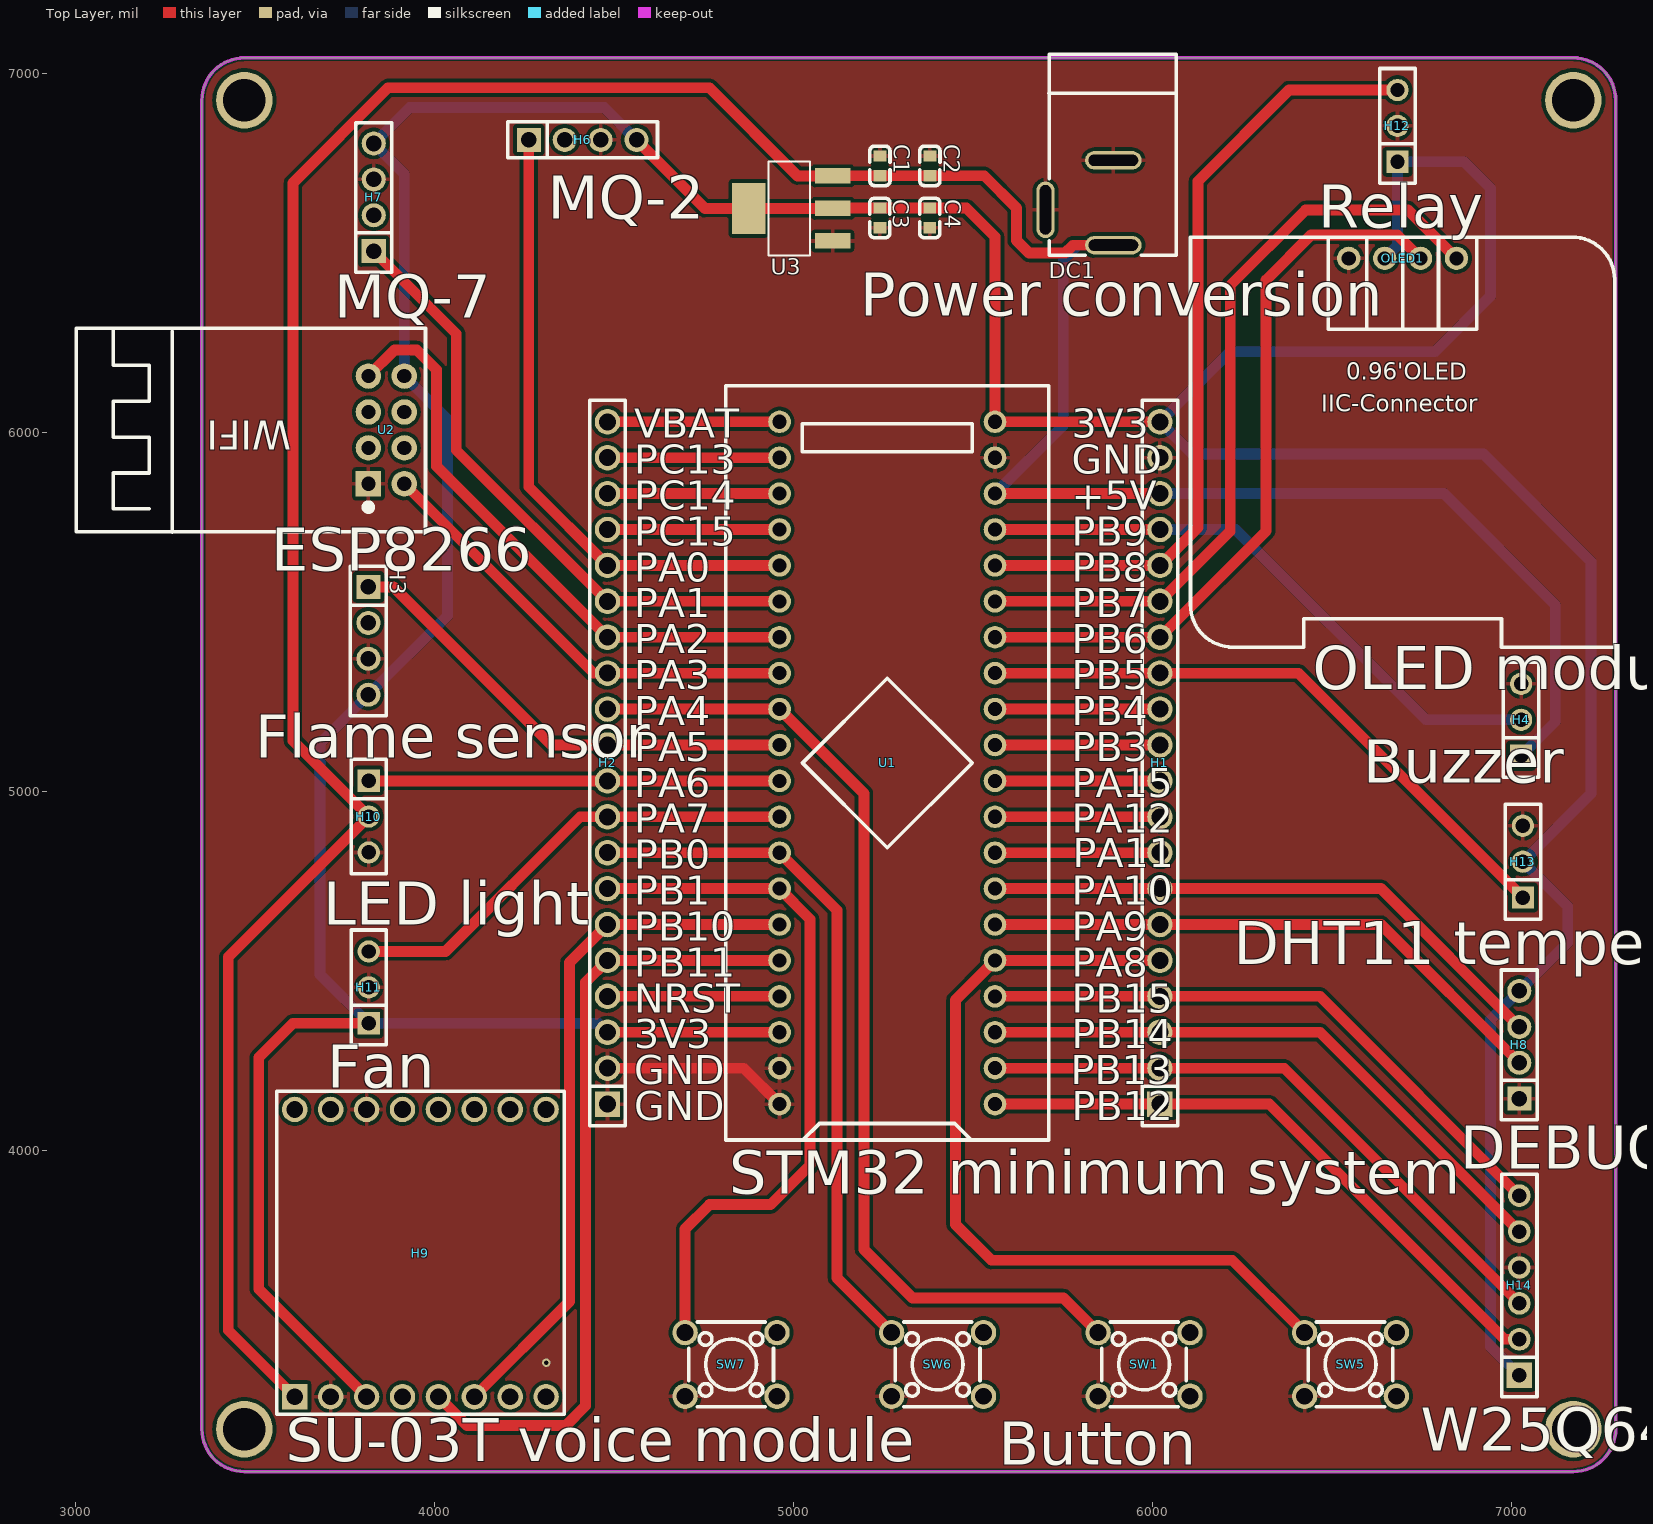
[diagram p0: Top Layer view]
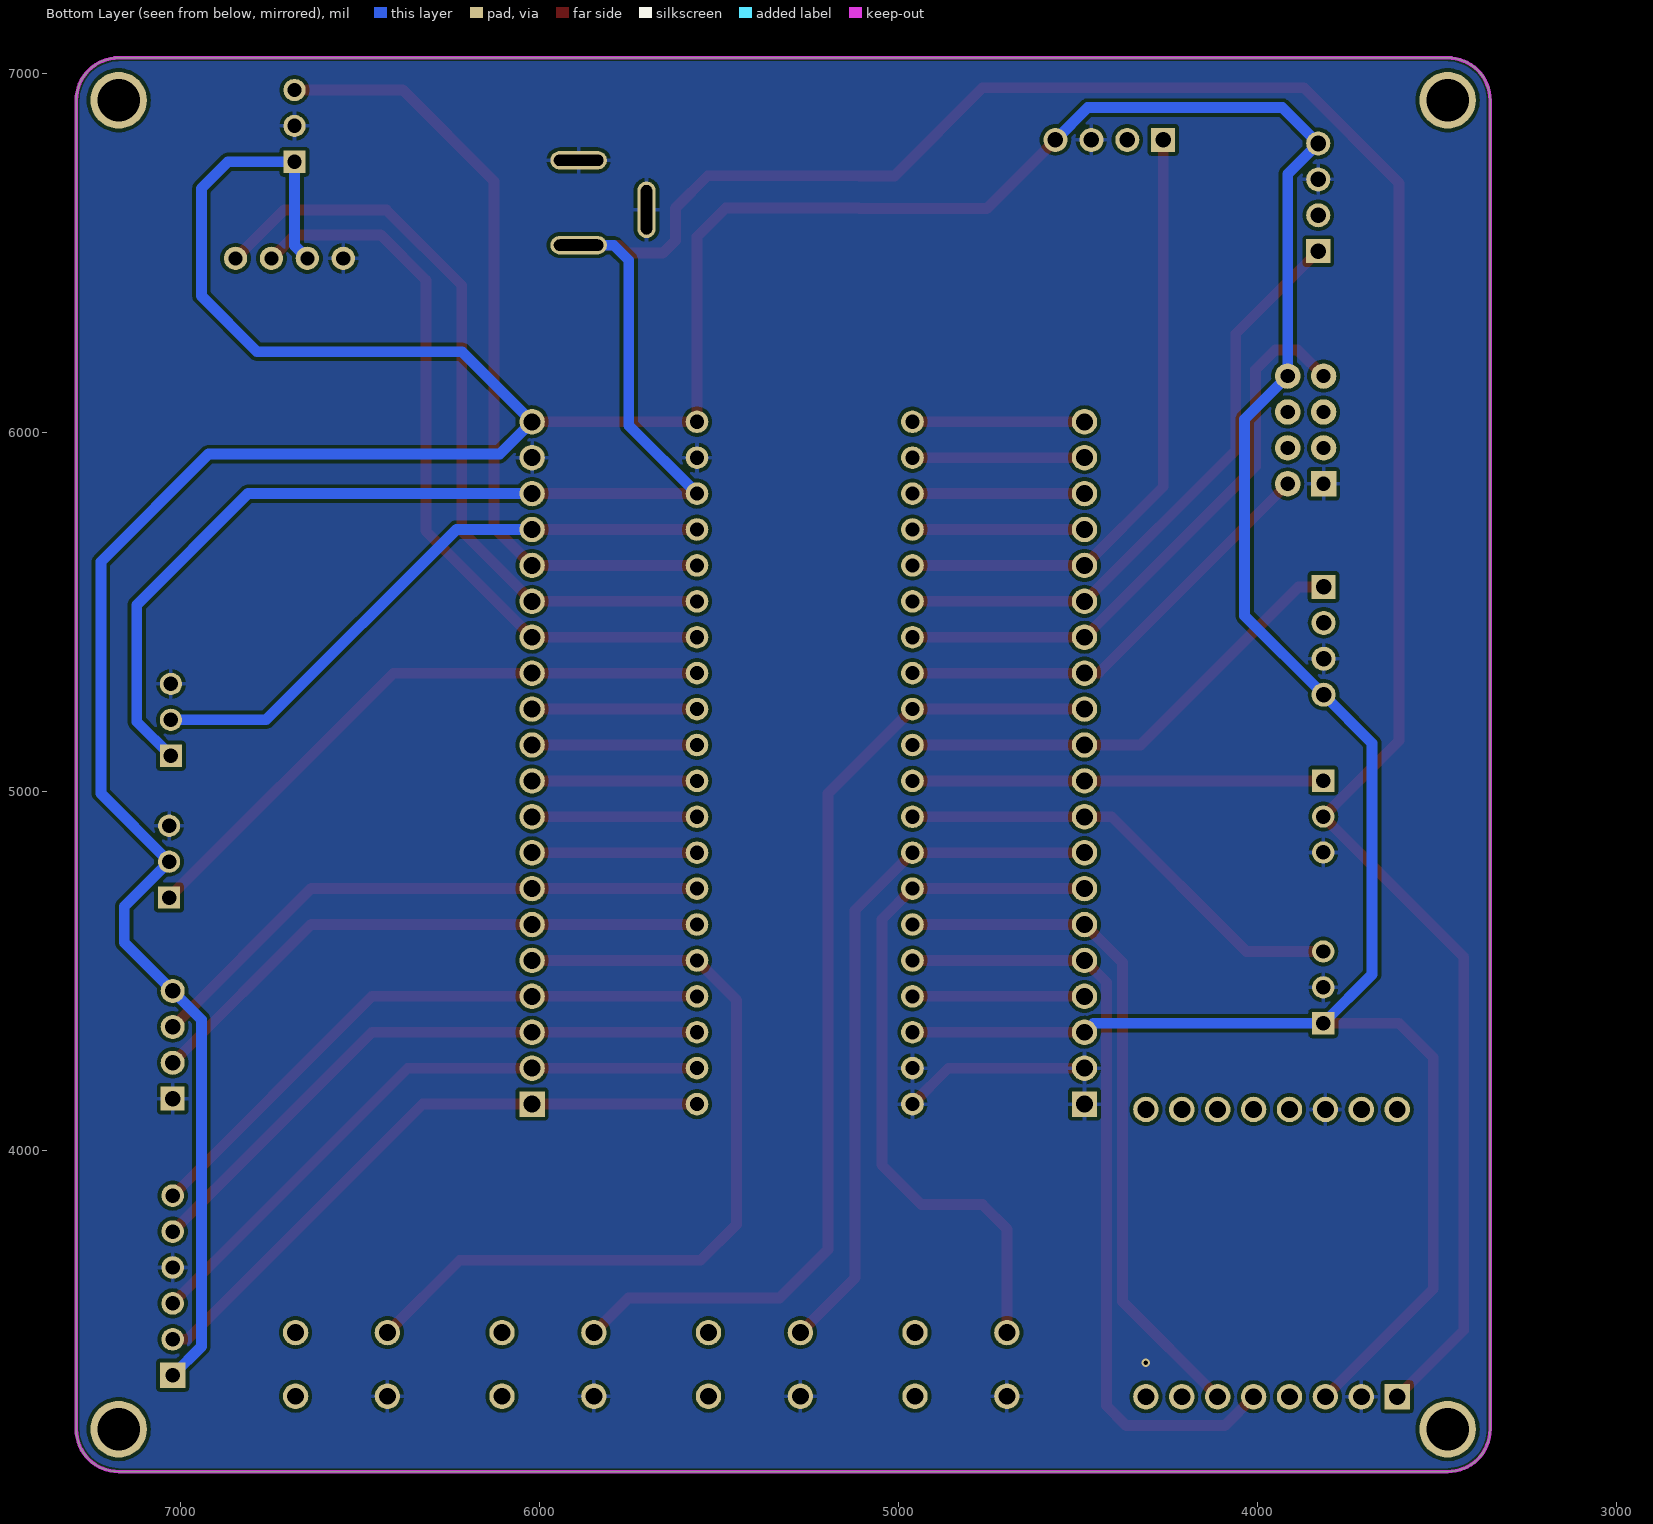
[diagram p1: Bottom Layer view, seen from below]
# Altium PCB MISC51915.pcbdoc
Units mil, origin at the board's own origin, x right, y up, seen from the top; angles counter-clockwise.
Board outline 3937.01 x 3937.01 mil, 2 copper layers (Top Layer, Bottom Layer), stack 62.206 mil thick; 26 components, 37 nets, 180 pads, 1 vias.

## Layer stack, top to bottom
Top Solder Mask Layer: solder mask 0.394, Dk 3.3
Top Layer: signal copper 1.379
Dielectric1: surface 59.449, FR4, Dk 4.5
Bottom Layer: signal copper 1.378
Bottom Solder Mask Layer: solder mask 0.394, Dk 3.3

## Board outline
3470.35,7043.5 ccw(c3470.35,6925.39) 3352.24,6925.39 3352.24,3224.61 ccw(c3470.35,3224.61) 3470.35,3106.5 7171.14,3106.5 ccw(c7171.14,3224.61) 7289.25,3224.61 7289.25,6925.39 ccw(c7171.14,6925.39) 7171.14,7043.5 3470.35,7043.5

## Design rules (kind name [scope] priority, off if disabled: settings)
BoardOutlineClearance copperThickness2oz_1 [All] p2 off: genericclearance=7.99 ignorepadtopadclearanceinfootprint=FALSE except(0: Arc-SplitContinuation Track-SplitContinuation SMDPad-SplitContinuation THPad-SplitContinuation Via-SplitContinuation Fill-SplitContinuation Region-SplitContinuation Poly-SplitContinuation Text-SplitContinuation Hole-SplitContinuation; 5.98: Arc-CutoutEdge Track-CutoutEdge SMDPad-CutoutEdge THPad-CutoutEdge Via-CutoutEdge Text-CutoutEdge; 6.9: Hole-OutlineEdge Hole-CutoutEdge; 10: Poly-OutlineEdge Poly-CutoutEdge; 11.81: Arc-OutlineEdge Track-OutlineEdge SMDPad-OutlineEdge THPad-OutlineEdge Via-OutlineEdge Fill-OutlineEdge Region-OutlineEdge Text-OutlineEdge Fill-CutoutEdge Region-CutoutEdge)
BoardOutlineClearance Plane_innerPlane_1 [All] p4 off: genericclearance=4.02 ignorepadtopadclearanceinfootprint=FALSE except(0: Arc-SplitContinuation Track-SplitContinuation SMDPad-SplitContinuation THPad-SplitContinuation Via-SplitContinuation Fill-SplitContinuation Region-SplitContinuation Poly-SplitContinuation Text-SplitContinuation Hole-SplitContinuation; 5.98: Arc-CutoutEdge Track-CutoutEdge SMDPad-CutoutEdge THPad-CutoutEdge Via-CutoutEdge Text-CutoutEdge; 6.9: Hole-OutlineEdge Hole-CutoutEdge; 10: Poly-OutlineEdge Poly-CutoutEdge; 11.81: Arc-OutlineEdge Track-OutlineEdge SMDPad-OutlineEdge THPad-OutlineEdge Via-OutlineEdge Fill-OutlineEdge Region-OutlineEdge Text-OutlineEdge Fill-CutoutEdge Region-CutoutEdge)
BoardOutlineClearance Copper_copperRegion_1 [All] p6 off: genericclearance=4.02 ignorepadtopadclearanceinfootprint=FALSE except(0: Arc-SplitContinuation Track-SplitContinuation SMDPad-SplitContinuation THPad-SplitContinuation Via-SplitContinuation Fill-SplitContinuation Region-SplitContinuation Poly-SplitContinuation Text-SplitContinuation Hole-SplitContinuation; 5.98: Arc-CutoutEdge Track-CutoutEdge SMDPad-CutoutEdge THPad-CutoutEdge Via-CutoutEdge Text-CutoutEdge; 6.9: Hole-OutlineEdge Hole-CutoutEdge; 10: Poly-OutlineEdge Poly-CutoutEdge; 11.81: Arc-OutlineEdge Track-OutlineEdge SMDPad-OutlineEdge THPad-OutlineEdge Via-OutlineEdge Fill-OutlineEdge Region-OutlineEdge Text-OutlineEdge Fill-CutoutEdge Region-CutoutEdge)
BoardOutlineClearance copperThickness1oz_1 [All] p8: genericclearance=4.02 ignorepadtopadclearanceinfootprint=FALSE except(0: Arc-SplitContinuation Track-SplitContinuation SMDPad-SplitContinuation THPad-SplitContinuation Via-SplitContinuation Fill-SplitContinuation Region-SplitContinuation Poly-SplitContinuation Text-SplitContinuation Hole-SplitContinuation; 5.98: Arc-CutoutEdge Track-CutoutEdge SMDPad-CutoutEdge THPad-CutoutEdge Via-CutoutEdge Text-CutoutEdge; 6.9: Hole-OutlineEdge Hole-CutoutEdge; 10: Poly-OutlineEdge Poly-CutoutEdge; 11.81: Arc-OutlineEdge Track-OutlineEdge SMDPad-OutlineEdge THPad-OutlineEdge Via-OutlineEdge Fill-OutlineEdge Region-OutlineEdge Text-OutlineEdge Fill-CutoutEdge Region-CutoutEdge)
Clearance copperThickness2oz [All] p1 off: gap=7.99 ignorepadtopadclearanceinfootprint=FALSE except(5.98: SMDPad-Track SMDPad-SMDPad THPad-Track SMDPad-THPad THPad-THPad Track-Via SMDPad-Via THPad-Via Via-Via Fill-SMDPad Region-SMDPad Fill-THPad Region-THPad Fill-Via Region-Via Fill-Fill Fill-Region Region-Region Arc-Track Arc-SMDPad Arc-THPad Arc-Via Fill-Arc Region-Arc Arc-Arc Text-Track SMDPad-Text Text-THPad Text-Via Fill-Text Region-Text Arc-Text Text-Text; 6.9: Hole-Track Hole-SMDPad Hole-THPad Hole-Via Fill-Hole Region-Hole Hole-Arc Hole-Text; 10: Poly-Track Poly-SMDPad Poly-THPad Poly-Via Poly-Fill Poly-Region Poly-Poly Poly-Arc Poly-Text Poly-Hole; 11.81: Fill-Track Region-Track)
Clearance Plane_innerPlane [All] p3 off: gap=4.02 ignorepadtopadclearanceinfootprint=FALSE except(5.98: SMDPad-Track SMDPad-SMDPad THPad-Track SMDPad-THPad THPad-THPad Track-Via SMDPad-Via THPad-Via Via-Via Fill-SMDPad Region-SMDPad Fill-THPad Region-THPad Fill-Via Region-Via Fill-Fill Fill-Region Region-Region Arc-Track Arc-SMDPad Arc-THPad Arc-Via Fill-Arc Region-Arc Arc-Arc Text-Track SMDPad-Text Text-THPad Text-Via Fill-Text Region-Text Arc-Text Text-Text; 6.9: Hole-Track Hole-SMDPad Hole-THPad Hole-Via Fill-Hole Region-Hole Hole-Arc Hole-Text; 10: Poly-Track Poly-SMDPad Poly-THPad Poly-Via Poly-Fill Poly-Region Poly-Poly Poly-Arc Poly-Text Poly-Hole; 11.81: Fill-Track Region-Track)
Clearance Copper_copperRegion [All] p5 off: gap=4.02 ignorepadtopadclearanceinfootprint=FALSE except(5.98: SMDPad-Track SMDPad-SMDPad THPad-Track SMDPad-THPad THPad-THPad Track-Via SMDPad-Via THPad-Via Via-Via Fill-SMDPad Region-SMDPad Fill-THPad Region-THPad Fill-Via Region-Via Fill-Fill Fill-Region Region-Region Arc-Track Arc-SMDPad Arc-THPad Arc-Via Fill-Arc Region-Arc Arc-Arc Text-Track SMDPad-Text Text-THPad Text-Via Fill-Text Region-Text Arc-Text Text-Text; 6.9: Hole-Track Hole-SMDPad Hole-THPad Hole-Via Fill-Hole Region-Hole Hole-Arc Hole-Text; 10: Poly-Track Poly-SMDPad Poly-THPad Poly-Via Poly-Fill Poly-Region Poly-Poly Poly-Arc Poly-Text Poly-Hole; 11.81: Fill-Track Region-Track)
Clearance copperThickness1oz [All] p7: gap=4.02 ignorepadtopadclearanceinfootprint=FALSE except(5.98: SMDPad-Track SMDPad-SMDPad THPad-Track SMDPad-THPad THPad-THPad Track-Via SMDPad-Via THPad-Via Via-Via Fill-SMDPad Region-SMDPad Fill-THPad Region-THPad Fill-Via Region-Via Fill-Fill Fill-Region Region-Region Arc-Track Arc-SMDPad Arc-THPad Arc-Via Fill-Arc Region-Arc Arc-Arc Text-Track SMDPad-Text Text-THPad Text-Via Fill-Text Region-Text Arc-Text Text-Text; 6.9: Hole-Track Hole-SMDPad Hole-THPad Hole-Via Fill-Hole Region-Hole Hole-Arc Hole-Text; 10: Poly-Track Poly-SMDPad Poly-THPad Poly-Via Poly-Fill Poly-Region Poly-Poly Poly-Arc Poly-Text Poly-Hole; 11.81: Fill-Track Region-Track)
DiffPairsRouting differentialPair [All] p1: maxlimit=6 minlimit=6 mostfreqgap=6 toplayer_minwidth=5 toplayer_prefwidth=10 toplayer_maxwidth=100 toplayer_mingap=6 toplayer_prefgap=6 toplayer_maxgap=6 bottomlayer_minwidth=5 bottomlayer_prefwidth=10 bottomlayer_maxwidth=100 bottomlayer_mingap=6 bottomlayer_prefgap=6 bottomlayer_maxgap=6 maxuncoupledlength=10
HoleToHoleClearance otherClearance [All] p1: gap=11.81 allowstackedmicrovias=TRUE
Length netLength [All] p1: minlimit=0 maxlimit=0
PasteMaskExpansion pasteMaskExpansion [All] p1: expansion=0
PlaneConnect innerPlane [All] p1: planeconnectstyle=Relief reliefexpansion=20 reliefentries=4 reliefconductorwidth=10 reliefairgap=10
PolygonConnect copperRegion [All] p1: connectstyle=Relief reliefconductorwidth=10 reliefentries=4 polygonreliefangle="90 Angle" airgapwidth=10 via.connectstyle=Relief via.reliefconductorwidth=10 via.reliefentries=4 via.polygonreliefangle="90 Angle" via.airgapwidth=10
RoutingVias viaSize [All] p1: holewidth=12.01 width=24.02 viastyle="Through Hole" minholewidth=11.81 minwidth=19.68 maxholewidth=248.03 maxwidth=393.7
SolderMaskExpansion solderMaskExpansion [IsVia] p1: expansion=-1000 istentingtop=TRUE
SolderMaskExpansion solderMaskExpansion [All] p2: expansion=2 istentingtop=FALSE
Width copperThickness2oz_2 [All] p1 off: maxlimit=100 minlimit=8 preferedwidth=10
Width copperThickness1oz_2 [All] p2: maxlimit=100 minlimit=5 preferedwidth=10

## Components (designator, comment, footprint, x,y, rotation, side; value= is the part's Value field where it differs from the comment)
C1 "100nF" C0603 5240.36,6742.51 r270 top
C2 "100nF" C0603 5379.49,6742.51 r270 top
C3 "100nF" C0603 5240.19,6597.5 r90 top
C4 "100nF" C0603 5379.32,6597.5 r90 top
DC1 "" DC-2.0 5900.75,6645 r90 top
H1 "" HDR-TH_20P-P2.54-V-F 6019.91,5080 r90 top
H2 "" HDR-TH_20P-P2.54-V-F 4481.7,5080 r90 top
H3 "" HDR-TH_4P-P2.54-V-F 3815.75,5420 r270 top
H4 "" HDR-TH_3P-P2.54-V-F 7025.75,5200 r90 top
H6 "" HDR-TH_4P-P2.54-V-F 4412.53,6815 r0 top
H7 "" HDR-TH_4P-P2.54-V-F 3830.75,6655 r90 top
H8 "" HDR-TH_4P-P2.54-V-F 7020.75,4295 r90 top
H9 "" HDR-TH_16P-P2.54-V-M-R2-C8-S2.54 3910.75,3315 r0 top
H10 "" HDR-TH_3P-P2.54-V-F 3816.75,4930.71 r270 top
H11 "" HDR-TH_3P-P2.54-V-F 3816.75,4455 r90 top
H12 "" HDR-TH_3P-P2.54-V-F 6681.51,6853.84 r90 top
H13 "" HDR-TH_3P-P2.54-V-F 7030.75,4805 r90 top
H14 "" HDR-TH_6P-P2.54-V-F 7020.75,3625 r90 top
OLED1 "" 0.96OLED_4P 6695.75,6485 r0 top
SW1 "" SW-TH_4P-L6.0-W6.0-P4.50-LS6.5 5975.75,3405 r0 top
SW5 "" SW-TH_4P-L6.0-W6.0-P4.50-LS6.5 6550.75,3405 r0 top
SW6 "" SW-TH_4P-L6.0-W6.0-P4.50-LS6.5 5400.75,3405 r0 top
SW7 "" SW-TH_4P-L6.0-W6.0-P4.50-LS6.5 4825.75,3405 r0 top
U1 "STM32F103C8T6-Card" CONN-TH_L53.3-W22.9_STM32F103C8T6-CARD 5260.75,5080 r90 top
U2 "Ai-Thinker ESP-01S ESP8266" WIFIM-TH_8P-L24.7-W14.4-P2.54 3865.75,6007.3 r180 top
U3 "AMS1117-3.3" SOT-223-3_L6.5-W3.4-P2.30-LS7.0-BR 4991.9,6624.1 r0 top

## Footprints (in the part's own frame and the unit in brackets; to place one, negate y for a bottom-side part, rotate by r counter-clockwise, add the part's x,y. Pads: shape width x height; smd on the part's side, far side on the other; paste and mask are expansions set on the pad)
0.96OLED_4P [mm]
  round 1.65 hole 1 copper offset 0,0: 1(-3.81,-0.001) 2(-1.27,0.002) 3(1.27,0.002) 4(3.81,0.002)
  silkscreen extent -15,-27.5 15,1.5
C0603 [mm]
  rect 0.8x0.9 smd: 1(-0.7,0) 2(0.7,0)
  silkscreen extent -1.39,-0.71 1.39,0.71
CONN-TH_L53.3-W22.9_STM32F103C8T6-CARD [mm]
  round 1.6 hole 1: 1(-24.13,-7.62) 2(-21.59,-7.62) 3(-19.05,-7.62) 4(-16.51,-7.62) 5(-13.97,-7.62) 6(-11.43,-7.62) 7(-8.89,-7.62) 8(-6.35,-7.62) 9(-3.81,-7.62) 10(-1.27,-7.62) 11(1.27,-7.62) 12(3.81,-7.62) 13(6.35,-7.62) 14(8.89,-7.62) 15(11.43,-7.62) 16(13.97,-7.62) 17(16.51,-7.62) 18(19.05,-7.62) 19(21.59,-7.62) 20(24.13,-7.62) 21(24.13,7.62) 22(21.59,7.62) 23(19.05,7.62) 24(16.51,7.62) 25(13.97,7.62) 26(11.43,7.62) 27(8.89,7.62) 28(6.35,7.62) 29(3.81,7.62) 30(1.27,7.62) 31(-1.27,7.62) 32(-3.81,7.62) 33(-6.35,7.62) 34(-8.89,7.62) 35(-11.43,7.62) 36(-13.97,7.62) 37(-16.51,7.62) 38(-19.05,7.62) 39(-21.59,7.62) 40(-24.13,7.62)
  silkscreen extent -26.67,-11.43 26.67,11.43
DC-2.0 [mil]
  oval 157.5x51.2 hole 31.5 slot 137.8 at 0 deg paste+0 mask+2: 2(-24.7,199.5)
  oval 51.2x157.5 hole 31.5 slot 137.8 at 90 deg paste+0 mask+2: 3(113.1,10.5) 4(-123.1,10.5)
  silkscreen extent -151,-165 408,190
HDR-TH_3P-P2.54-V-F [mil]
  rect 62x62 hole 40.16: 1(-100,0)
  round 62 hole 40.16: 2(0,0) 3(100,0)
  silkscreen extent -160,-49 160,49
HDR-TH_4P-P2.54-V-F [mm]
  rect 1.7x1.7 hole 1.1: 1(-3.81,0)
  round 1.7 hole 1.1: 2(-1.27,0) 3(1.27,0) 4(3.81,0)
  silkscreen extent -5.29,-1.27 5.29,1.27
HDR-TH_6P-P2.54-V-F [mm]
  rect 1.8x1.8 hole 1.02: 1(-6.35,0)
  round 1.6 hole 1.02: 2(-3.81,0) 3(-1.27,0) 4(1.27,0) 5(3.81,0) 6(6.35,0)
  silkscreen extent -7.87,-1.25 7.87,1.25
HDR-TH_16P-P2.54-V-M-R2-C8-S2.54 [mm]
  rect 1.8x1.8 hole 1.2: 1(-7.62,0)
  round 1.8 hole 1.2: 2(-7.62,20.32) 3(-5.08,0) 4(-5.08,20.32) 5(-2.54,0) 6(-2.54,20.32) 7(0,0) 8(0,20.32) 9(2.54,0) 10(2.54,20.32) 11(5.08,0) 12(5.08,20.32) 13(7.62,0) 14(7.62,20.32) 15(10.16,0) 16(10.16,20.32)
  silkscreen extent -8.89,-1.23 11.43,21.6
HDR-TH_20P-P2.54-V-F [mm]
  rect 1.8x1.8 hole 1.2: 1(-24.13,0)
  round 1.8 hole 1.2: 2(-21.59,0) 3(-19.05,0) 4(-16.51,0) 5(-13.97,0) 6(-11.43,0) 7(-8.89,0) 8(-6.35,0) 9(-3.81,0) 10(-1.27,0) 11(1.27,0) 12(3.81,0) 13(6.35,0) 14(8.89,0) 15(11.43,0) 16(13.97,0) 17(16.51,0) 18(19.05,0) 19(21.59,0) 20(24.13,0)
  silkscreen extent -25.65,-1.25 25.65,1.25
SOT-223-3_L6.5-W3.4-P2.30-LS7.0-BR [mm]
  rect 2.5x1.1 smd: 1(2.97,-2.3) 2(2.97,0) 3(2.97,2.3)
  rect 2.34x3.6 smd: 4(-2.97,0)
  silkscreen extent -1.57,-3.33 1.37,3.33
SW-TH_4P-L6.0-W6.0-P4.50-LS6.5 [mm]
  round 1.8 hole 1.2: 1(-3.25,2.25) 2(3.25,2.25) 3(-3.25,-2.25) 4(3.25,-2.25)
  silkscreen extent -3,-3 3,3
WIFIM-TH_8P-L24.7-W14.4-P2.54 [mm]
  rect 1.8x1.8 hole 1 paste+0 mask+0.05: 1(1.27,3.81)
  round 1.8 hole 1 paste+0 mask+0.05: 2(1.27,1.27) 3(1.27,-1.27) 4(1.27,-3.81) 5(-1.27,3.81) 6(-1.27,1.27) 7(-1.27,-1.27) 8(-1.27,-3.81)
  silkscreen extent -2.77,-7.19 21.93,7.24

## Free pads (board coordinates)
  round 157.48 hole 118.11: 1(3470.35,6925.39) 1(3470.35,3224.61) 1(7171.14,6925.39) 1(7171.14,3224.61)

## Via types
v1: diameter 24.02, hole 12, Top Layer to Bottom Layer, 1 vias

## Nets (pads, with @x,y where several pads share a name; then routed paths per layer and width w, separated by ;. In a path a pad name is that pad's centre, name@x,y a point inside that pad or via, vN(x,y) a via of type N, cw(c..) or ccw(c..) an arc to the next point about the centre after c; other vN are vias at no path point)
+5V: C1.2 C2.2 DC1.4 H1.18 H4.1 H9.1 H10.2 U1.18 U3.3 | length 9386.1
  Top Layer w30: H9.1 3425.75,3500 3425.75,4539.71 H10.2 3605.75,5141.71 3605.75,6695 3870.75,6960 4765.75,6960 5011.1,6714.65 U3.3 5109.12,6714.95 C1.2 C2.2 5530.8,6714.95 5620.75,6625 5620.75,6535 5655.75,6500 5755.75,6500 5777.65,6521.9 DC1.4 ; U1.18 H1.18
  Bottom Layer w30: U1.18 5750.75,6020 5750.75,6480 5792.65,6521.9 DC1.4 ; H1.18 6810.75,5830 7120.75,5520 7120.75,5195 H4.1
GND: C1.1 C2.1 C3.1 C4.1 DC1.2 DC1.3 H1.19 H2.1 H2.2 H3.3 H4.3 H6.3 H7.3 H8.1 H9.3 H9.6 H10.3 H11.2 H12.2 H13.3 H14.4 OLED1.1 SW1.3 SW5.3 SW6.3 SW7.3 U1.19 U1.39 U1.40 U2.1 U3.1 | length 520.5
  Top Layer w30: H2.2 4860.74,4230 U1.40
  other v1: 4310.75,3410
NRST: H2.4 U1.37 | length 479
  Top Layer w30: H2.4 U1.37
PA0: H2.16 H6.1 U1.25 | length 1754.8
  Top Layer w30: H6.1 4262.53,5849.16 H2.16 U1.25
PA1: H2.15 H7.1 U1.26 | length 1723.7
  Top Layer w30: H7.1 4060.75,6275 4060.75,5950.95 H2.15 U1.26
PA2: H2.14 U1.27 U2.4 | length 1664.1
  Top Layer w30: U2.4 3888.44,6230 3950.75,6230 4005.75,6175 4005.75,5905.95 H2.14 U1.27
PA3: H2.13 U1.28 U2.5 | length 1263.4
  Top Layer w30: U2.5 4443.05,5330 H2.13 U1.28
PA4: H2.12 SW1.1 U1.29 | length 2829.3
  Top Layer w30: H2.12 U1.29 5195.75,4995 5195.75,3725 5330.75,3590 5751.38,3590 SW1.1
PA5: H2.11 H3.1 U1.30 | length 1327.3
  Top Layer w30: H3.1 3885.75,5570 4325.74,5130 H2.11 U1.30
PA6: H2.10 H10.1 U1.31 | length 1144.3
  Top Layer w30: H10.1 3817.46,5030 H2.10 U1.31
PA7: H2.9 H11.3 U1.32 | length 1299.3
  Top Layer w30: H11.3 4030.75,4555 4405.75,4930 H2.9 U1.32
PA8: H1.5 SW5.1 U1.5 | length 2336.6
  Top Layer w30: H1.5 U1.5 5450.75,4420 5450.75,3795 5550.75,3695 6221.38,3695 SW5.1
PA9: H1.6 H8.2 U1.6 | length 1619.5
  Top Layer w30: U1.6 H1.6 6635.75,4630 H8.2
PA10: H1.7 H8.3 U1.7 | length 1619.5
  Top Layer w30: U1.7 H1.7 6635.75,4730 H8.3
PA11: H1.8 U1.8 | length 459.2
  Top Layer w30: U1.8 H1.8
PA12: H1.9 U1.9 | length 459.2
  Top Layer w30: U1.9 H1.9
PA15: H1.10 U1.10 | length 459.2
  Top Layer w30: U1.10 H1.10
PB0: H2.8 SW6.1 U1.33 | length 1944.7
  Top Layer w30: H2.8 U1.33 5120.75,4670 5120.75,3645.63 SW6.1
PB1: H2.7 SW7.1 U1.34 | length 1994.4
  Top Layer w30: H2.7 U1.34 5045.75,4645 5045.75,3960 4935.75,3850 4765.75,3850 4697.8,3782.05 SW7.1
PB3: H1.11 U1.11 | length 459.2
  Top Layer w30: U1.11 H1.11
PB4: H1.12 U1.12 | length 459.2
  Top Layer w30: U1.12 H1.12
PB5: H1.13 H13.1 U1.13 | length 1728.9
  Top Layer w30: U1.13 H1.13 6405.75,5330 H13.1
PB6: H1.14 OLED1.3 U1.14 | length 2085.4
  Top Layer w30: U1.14 H1.14 6315.75,5725.84 6315.75,6425 6440.75,6550 6680.8,6550 OLED1.3@6745.75,6485.05
PB7: H1.15 OLED1.4 U1.15 | length 2193.2
  Top Layer w30: U1.15 H1.15 6215.75,5725.84 6215.75,6410 6425.75,6620 6710.8,6620 OLED1.4@6845.75,6485.05
PB8: H1.16 H12.3 U1.16 | length 2233.9
  Top Layer w30: U1.16 H1.16 6125.75,5735.84 6125.75,6700 6379.58,6953.84 H12.3
PB9: H1.17 H4.2 U1.17 | length 1684.5
  Top Layer w30: U1.17 H1.17
  Bottom Layer w30: H1.17 6230.75,5730 6760.75,5200 H4.2
PB10: H2.6 H9.11 U1.35 | length 1947.7
  Top Layer w30: H9.11 4375.75,3580 4375.75,4524.05 H2.6 U1.35
PB11: H2.5 H9.9 U1.36 | length 2210.2
  Top Layer w30: H9.9 4090.75,3235 4365.75,3235 4420.75,3290 4420.75,4469.05 H2.5 U1.36
PB12: H1.1 H14.2 U1.1 | length 1731.3
  Top Layer w30: U1.1 H1.1 6324.62,4130 6979.63,3475 H14.2
PB13: H1.2 H14.3 U1.2 | length 1731.5
  Top Layer w30: U1.2 H1.2 6366.05,4230 7020.75,3575.3 H14.3
PB14: H1.3 H14.5 U1.3 | length 1689.9
  Top Layer w30: U1.3 H1.3 6465.74,4330 H14.5
PB15: H1.4 H14.6 U1.4 | length 1689.9
  Top Layer w30: U1.4 H1.4 6465.74,4430 H14.6
PC13: H2.19 U1.22 | length 479
  Top Layer w30: H2.19 U1.22
PC14: H2.18 U1.23 | length 479
  Top Layer w30: H2.18 U1.23
PC15: H2.17 U1.24 | length 479
  Top Layer w30: H2.17 U1.24
VBAT: H2.20 U1.21 | length 479
  Top Layer w30: H2.20 U1.21
VCC: C3.2 C4.2 H1.20 H2.3 H3.4 H6.4 H7.4 H8.4 H9.5 H11.1 H12.1 H13.2 H14.1 OLED1.2 U1.20 U1.38 U2.8 U3.2 U3.4 | length 14022
  Top Layer w30: H9.5 3510.75,3615 3510.75,4260 3605.75,4355 H11.1 ; H2.3 U1.38 ; H6.4 4753.44,6624.1 U3.4 U3.2 5109.79,6625.06 C3.2 C4.2 5480.68,6625.06 5560.74,6545 U1.20 H1.20
  Bottom Layer w30: H2.3 4456.7,4355 H11.1 3680.75,4491 3680.75,5135 H3.4 4035.75,5490 4035.75,6037.3 U2.8 3915.75,6720 H7.4 3930.75,6905 4472.53,6905 H6.4 ; OLED1.2@6645.75,6485.05 6681.51,6520.81 H12.1 6866.91,6753.84 6940.75,6680 6940.75,6380 6785.75,6225 6214.91,6225 H1.20 6109.91,5940 6920.75,5940 7220.75,5640 7220.75,4995 H13.2 7155.75,4680 7155.75,4580 H8.4 6940.75,4365 6940.75,3455 H14.1
pads on no net: H3.2 H6.2 H7.2 H9.2 H9.4 H9.7 H9.8 H9.10 H9.12 H9.13 H9.14 H9.15 H9.16 SW1.2 SW1.4 SW5.2 SW5.4 SW6.2 SW6.4 SW7.2 SW7.4 U2.2 U2.3 U2.6 U2.7

## Polygon pours and split planes (outlines as drawn)
GND on Bottom Layer (solid, remove dead copper, pour order 2): 3280.75,7165 3280.75,3000 7455.75,3000 7455.75,7165
GND on Top Layer (solid, remove dead copper, pour order 0): 3180.75,7145 3180.75,3075 7565.75,3075 7565.75,7145

## Keep-outs
Board Outline Layer:
  the board outline again, w10

## Silkscreen, mask and mechanical layers (free items; w line width, h text height)
Top Silkscreen Layer:
  text "MQ-2" at 4315.75,6595 h120
  text "Relay" at 6460.75,6570 h120
  text "Power conversion" at 5185.75,6325 h120
  text "MQ-7" at 3720.75,6320 h120
  text "VBAT" at 4556.7,5985 h80
  text "3V3" at 5774.91,5985 h80
  text "PC13" at 4556.7,5885 h80
  text "GND" at 5774.91,5885 h80
  text "PC14" at 4556.7,5785 h80
  text "+5V" at 5774.91,5785 h80
  text "PC15" at 4556.7,5685 h80
  text "PB9" at 5774.91,5685 h80
  text "ESP8266" at 3545.75,5615 h120
  text "PA0" at 4556.7,5585 h80
  text "PB8" at 5774.91,5585 h80
  text "PA1" at 4556.7,5485 h80
  text "PB7" at 5774.91,5485 h80
  text "PA2" at 4556.7,5385 h80
  text "PB6" at 5774.91,5385 h80
  text "PA3" at 4556.7,5285 h80
  text "PB5" at 5774.91,5285 h80
  text "OLED module" at 6445.75,5285 h120
  text "PA4" at 4556.7,5185 h80
  text "PB4" at 5774.91,5185 h80
  text "Flame sensor" at 3500.75,5095 h120
  text "PA5" at 4556.7,5085 h80
  text "PB3" at 5774.91,5085 h80
  text "Buzzer" at 6585.75,5025 h120
  text "PA6" at 4556.7,4985 h80
  text "PA15" at 5774.91,4985 h80
  text "PA7" at 4556.7,4885 h80
  text "PA12" at 5774.91,4885 h80
  text "PA11" at 5776.7,4790 h80
  text "PB0" at 4556.7,4785 h80
  text "PB1" at 4556.7,4685 h80
  text "PA10" at 5774.91,4685 h80
  text "LED light" at 3690.75,4630 h120
  text "PB10" at 4556.7,4585 h80
  text "PA9" at 5774.91,4585 h80
  text "DHT11 temperature and humidity sensor" at 6225.75,4520 h120
  text "PB11" at 4556.7,4485 h80
  text "PA8" at 5774.91,4485 h80
  text "NRST" at 4556.7,4385 h80
  text "PB15" at 5774.91,4385 h80
  text "3V3" at 4556.7,4285 h80
  text "PB14" at 5774.91,4285 h80
  text "GND" at 4556.7,4185 h80
  text "PB13" at 5771.7,4185 h80
  text "Fan" at 3700.75,4175 h120
  text "GND" at 4556.7,4085 h80
  text "PB12" at 5774.91,4085 h80
  text "DEBUG" at 6855.75,3950 h120
  text "STM32 minimum system" at 4820.75,3880 h120
  text "W25Q64" at 6745.75,3165 h120
  text "SU-03T voice module" at 3585.75,3135 h120
  text "Button" at 5570.75,3125 h120